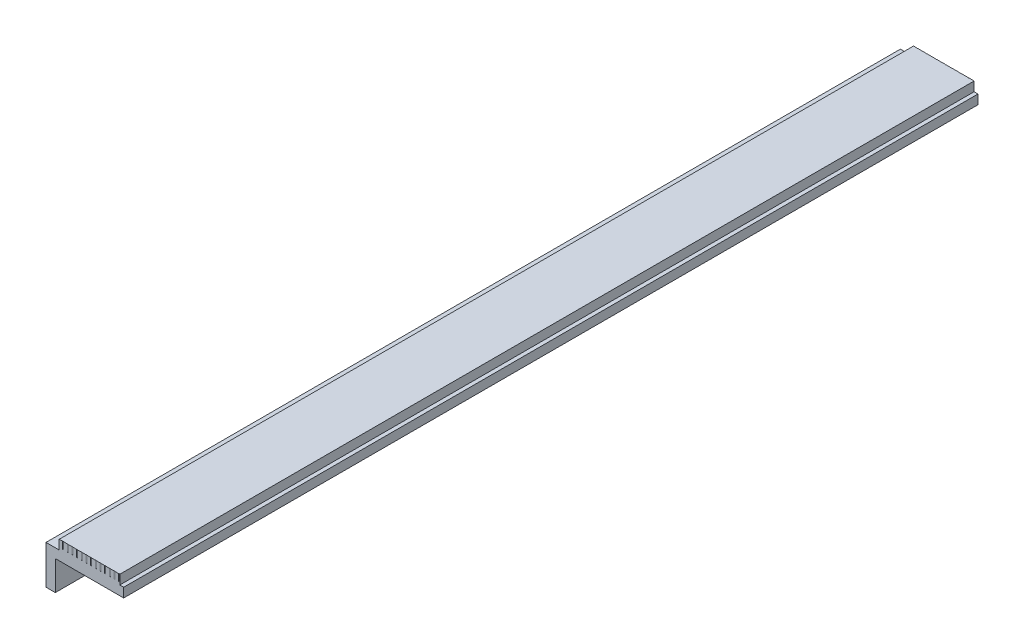
from build123d import *

# Parameters (mm, degrees)
BOSS_EXTRUDE1_DEPTH      = 1100
SKETCH2_W                = 1.259860676
SKETCH2_H                = 9.043092937
CUT_EXTRUDE1_DEPTH       = 0.2
LPATTERN1_COUNT          = 16
LPATTERN1_PITCH          = 6
MIRROR1_COPY_1_SKETCH_W  = 1.259860676
MIRROR1_COPY_1_SKETCH_H  = 9.043092937
MIRROR1_COPY_1_DEPTH     = 0.2
MIRROR1_COPY_2_SKETCH_W  = 1.259860676
MIRROR1_COPY_2_SKETCH_H  = 9.043092937
MIRROR1_COPY_2_DEPTH     = 0.2
MIRROR1_COPY_3_SKETCH_W  = 1.259860676
MIRROR1_COPY_3_SKETCH_H  = 9.043092937
MIRROR1_COPY_3_DEPTH     = 0.2
MIRROR1_COPY_4_SKETCH_W  = 1.259860676
MIRROR1_COPY_4_SKETCH_H  = 9.043092937
MIRROR1_COPY_4_DEPTH     = 0.2
MIRROR1_COPY_5_SKETCH_W  = 1.259860676
MIRROR1_COPY_5_SKETCH_H  = 9.043092937
MIRROR1_COPY_5_DEPTH     = 0.2
MIRROR1_COPY_6_SKETCH_W  = 1.259860676
MIRROR1_COPY_6_SKETCH_H  = 9.043092937
MIRROR1_COPY_6_DEPTH     = 0.2
MIRROR1_COPY_7_SKETCH_W  = 1.259860676
MIRROR1_COPY_7_SKETCH_H  = 9.043092937
MIRROR1_COPY_7_DEPTH     = 0.2
MIRROR1_COPY_8_SKETCH_W  = 1.259860676
MIRROR1_COPY_8_SKETCH_H  = 9.043092937
MIRROR1_COPY_8_DEPTH     = 0.2
MIRROR1_COPY_9_SKETCH_W  = 1.259860676
MIRROR1_COPY_9_SKETCH_H  = 9.043092937
MIRROR1_COPY_9_DEPTH     = 0.2
MIRROR1_COPY_10_SKETCH_W = 1.259860676
MIRROR1_COPY_10_SKETCH_H = 9.043092937
MIRROR1_COPY_10_DEPTH    = 0.2
MIRROR1_COPY_11_SKETCH_W = 1.259860676
MIRROR1_COPY_11_SKETCH_H = 9.043092937
MIRROR1_COPY_11_DEPTH    = 0.2
MIRROR1_COPY_12_SKETCH_W = 1.259860676
MIRROR1_COPY_12_SKETCH_H = 9.043092937
MIRROR1_COPY_12_DEPTH    = 0.2
MIRROR1_COPY_13_SKETCH_W = 1.259860676
MIRROR1_COPY_13_SKETCH_H = 9.043092937
MIRROR1_COPY_13_DEPTH    = 0.2
MIRROR1_COPY_14_SKETCH_W = 1.259860676
MIRROR1_COPY_14_SKETCH_H = 9.043092937
MIRROR1_COPY_14_DEPTH    = 0.2
MIRROR1_COPY_15_SKETCH_W = 1.259860676
MIRROR1_COPY_15_SKETCH_H = 9.043092937
MIRROR1_COPY_15_DEPTH    = 0.2
SKETCH3_W                = 12
SKETCH3_H                = 50
BOSS_EXTRUDE2_DEPTH      = 1100
SKETCH4_W                = 12
SKETCH4_H                = 88
CUT_EXTRUDE2_DEPTH       = 1110.053650641


with BuildPart() as part:
    # Sketch1 → Boss-Extrude1 (new body)
    with BuildSketch(Plane.XY):
        Polygon((0, 0), (100, 0), (100, 12), (95, 12), (95, 24), (17, 24), (17, 12), (12, 12), (12, 100), (0, 100), align=None)
    extrude(amount=BOSS_EXTRUDE1_DEPTH)

    # Sketch2 → Cut-Extrude1 (cut)
    with BuildSketch(Plane.XY.offset(1100)):
        with Locations((22.109179897, 19.478453532)):
            Rectangle(SKETCH2_W, SKETCH2_H)
    cut_extrude1 = extrude(amount=-CUT_EXTRUDE1_DEPTH, mode=Mode.SUBTRACT)

    # LPattern1: Cut-Extrude1 ×16
    with Locations(*[(i * LPATTERN1_PITCH, 0, 0) for i in range(1, LPATTERN1_COUNT)]):
        add(cut_extrude1, mode=Mode.SUBTRACT)

    # Mirror1: Cut-Extrude1 across plane
    add(cut_extrude1.mirror(Plane(origin=(0, 0, 550), x_dir=(1, 0, 0), z_dir=(0, 0, -1))), mode=Mode.SUBTRACT)

    # Mirror1 copy 1 sketch → Mirror1 copy 1 (cut)
    with BuildSketch(Plane(origin=(6, 0, 0), x_dir=(1, 0, 0), z_dir=(0, 0, -1))):
        with Locations((22.109179897, -19.478453532)):
            Rectangle(MIRROR1_COPY_1_SKETCH_W, MIRROR1_COPY_1_SKETCH_H)
    extrude(amount=-MIRROR1_COPY_1_DEPTH, mode=Mode.SUBTRACT)

    # Mirror1 copy 2 sketch → Mirror1 copy 2 (cut)
    with BuildSketch(Plane(origin=(12, 0, 0), x_dir=(1, 0, 0), z_dir=(0, 0, -1))):
        with Locations((22.109179897, -19.478453532)):
            Rectangle(MIRROR1_COPY_2_SKETCH_W, MIRROR1_COPY_2_SKETCH_H)
    extrude(amount=-MIRROR1_COPY_2_DEPTH, mode=Mode.SUBTRACT)

    # Mirror1 copy 3 sketch → Mirror1 copy 3 (cut)
    with BuildSketch(Plane(origin=(18, 0, 0), x_dir=(1, 0, 0), z_dir=(0, 0, -1))):
        with Locations((22.109179897, -19.478453532)):
            Rectangle(MIRROR1_COPY_3_SKETCH_W, MIRROR1_COPY_3_SKETCH_H)
    extrude(amount=-MIRROR1_COPY_3_DEPTH, mode=Mode.SUBTRACT)

    # Mirror1 copy 4 sketch → Mirror1 copy 4 (cut)
    with BuildSketch(Plane(origin=(24, 0, 0), x_dir=(1, 0, 0), z_dir=(0, 0, -1))):
        with Locations((22.109179897, -19.478453532)):
            Rectangle(MIRROR1_COPY_4_SKETCH_W, MIRROR1_COPY_4_SKETCH_H)
    extrude(amount=-MIRROR1_COPY_4_DEPTH, mode=Mode.SUBTRACT)

    # Mirror1 copy 5 sketch → Mirror1 copy 5 (cut)
    with BuildSketch(Plane(origin=(30, 0, 0), x_dir=(1, 0, 0), z_dir=(0, 0, -1))):
        with Locations((22.109179897, -19.478453532)):
            Rectangle(MIRROR1_COPY_5_SKETCH_W, MIRROR1_COPY_5_SKETCH_H)
    extrude(amount=-MIRROR1_COPY_5_DEPTH, mode=Mode.SUBTRACT)

    # Mirror1 copy 6 sketch → Mirror1 copy 6 (cut)
    with BuildSketch(Plane(origin=(36, 0, 0), x_dir=(1, 0, 0), z_dir=(0, 0, -1))):
        with Locations((22.109179897, -19.478453532)):
            Rectangle(MIRROR1_COPY_6_SKETCH_W, MIRROR1_COPY_6_SKETCH_H)
    extrude(amount=-MIRROR1_COPY_6_DEPTH, mode=Mode.SUBTRACT)

    # Mirror1 copy 7 sketch → Mirror1 copy 7 (cut)
    with BuildSketch(Plane(origin=(42, 0, 0), x_dir=(1, 0, 0), z_dir=(0, 0, -1))):
        with Locations((22.109179897, -19.478453532)):
            Rectangle(MIRROR1_COPY_7_SKETCH_W, MIRROR1_COPY_7_SKETCH_H)
    extrude(amount=-MIRROR1_COPY_7_DEPTH, mode=Mode.SUBTRACT)

    # Mirror1 copy 8 sketch → Mirror1 copy 8 (cut)
    with BuildSketch(Plane(origin=(48, 0, 0), x_dir=(1, 0, 0), z_dir=(0, 0, -1))):
        with Locations((22.109179897, -19.478453532)):
            Rectangle(MIRROR1_COPY_8_SKETCH_W, MIRROR1_COPY_8_SKETCH_H)
    extrude(amount=-MIRROR1_COPY_8_DEPTH, mode=Mode.SUBTRACT)

    # Mirror1 copy 9 sketch → Mirror1 copy 9 (cut)
    with BuildSketch(Plane(origin=(54, 0, 0), x_dir=(1, 0, 0), z_dir=(0, 0, -1))):
        with Locations((22.109179897, -19.478453532)):
            Rectangle(MIRROR1_COPY_9_SKETCH_W, MIRROR1_COPY_9_SKETCH_H)
    extrude(amount=-MIRROR1_COPY_9_DEPTH, mode=Mode.SUBTRACT)

    # Mirror1 copy 10 sketch → Mirror1 copy 10 (cut)
    with BuildSketch(Plane(origin=(60, 0, 0), x_dir=(1, 0, 0), z_dir=(0, 0, -1))):
        with Locations((22.109179897, -19.478453532)):
            Rectangle(MIRROR1_COPY_10_SKETCH_W, MIRROR1_COPY_10_SKETCH_H)
    extrude(amount=-MIRROR1_COPY_10_DEPTH, mode=Mode.SUBTRACT)

    # Mirror1 copy 11 sketch → Mirror1 copy 11 (cut)
    with BuildSketch(Plane(origin=(66, 0, 0), x_dir=(1, 0, 0), z_dir=(0, 0, -1))):
        with Locations((22.109179897, -19.478453532)):
            Rectangle(MIRROR1_COPY_11_SKETCH_W, MIRROR1_COPY_11_SKETCH_H)
    extrude(amount=-MIRROR1_COPY_11_DEPTH, mode=Mode.SUBTRACT)

    # Mirror1 copy 12 sketch → Mirror1 copy 12 (cut)
    with BuildSketch(Plane(origin=(72, 0, 0), x_dir=(1, 0, 0), z_dir=(0, 0, -1))):
        with Locations((22.109179897, -19.478453532)):
            Rectangle(MIRROR1_COPY_12_SKETCH_W, MIRROR1_COPY_12_SKETCH_H)
    extrude(amount=-MIRROR1_COPY_12_DEPTH, mode=Mode.SUBTRACT)

    # Mirror1 copy 13 sketch → Mirror1 copy 13 (cut)
    with BuildSketch(Plane(origin=(78, 0, 0), x_dir=(1, 0, 0), z_dir=(0, 0, -1))):
        with Locations((22.109179897, -19.478453532)):
            Rectangle(MIRROR1_COPY_13_SKETCH_W, MIRROR1_COPY_13_SKETCH_H)
    extrude(amount=-MIRROR1_COPY_13_DEPTH, mode=Mode.SUBTRACT)

    # Mirror1 copy 14 sketch → Mirror1 copy 14 (cut)
    with BuildSketch(Plane(origin=(84, 0, 0), x_dir=(1, 0, 0), z_dir=(0, 0, -1))):
        with Locations((22.109179897, -19.478453532)):
            Rectangle(MIRROR1_COPY_14_SKETCH_W, MIRROR1_COPY_14_SKETCH_H)
    extrude(amount=-MIRROR1_COPY_14_DEPTH, mode=Mode.SUBTRACT)

    # Mirror1 copy 15 sketch → Mirror1 copy 15 (cut)
    with BuildSketch(Plane(origin=(90, 0, 0), x_dir=(1, 0, 0), z_dir=(0, 0, -1))):
        with Locations((22.109179897, -19.478453532)):
            Rectangle(MIRROR1_COPY_15_SKETCH_W, MIRROR1_COPY_15_SKETCH_H)
    extrude(amount=-MIRROR1_COPY_15_DEPTH, mode=Mode.SUBTRACT)

    # Sketch3 → Boss-Extrude2 (add)
    with BuildSketch(Plane.XY.offset(1100)):
        with Locations((6, -13)):
            Rectangle(SKETCH3_W, SKETCH3_H)
    extrude(amount=-BOSS_EXTRUDE2_DEPTH)

    # Sketch4 → Cut-Extrude2 (cut, through all)
    with BuildSketch(Plane.XY.offset(1100)):
        with Locations((6, 56)):
            Rectangle(SKETCH4_W, SKETCH4_H)
    extrude(amount=-CUT_EXTRUDE2_DEPTH, mode=Mode.SUBTRACT)


solid = part.part
